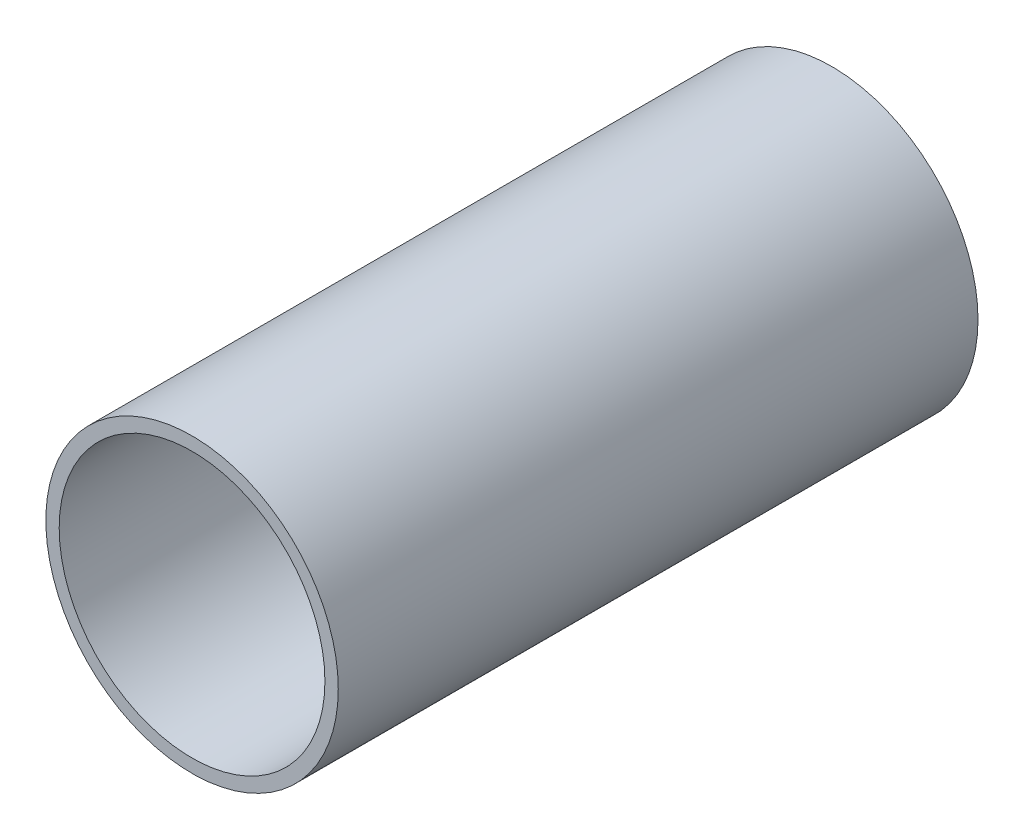
SolidWorks part; units mm, degrees
material "SPHC"
ref_plane "Front Plane" through (0, 0, 0) normal (0, 0, 1) x (1, 0, 0)
ref_plane "Top Plane" through (0, 0, 0) normal (0, 1, 0) x (1, 0, 0)
ref_plane "Right Plane" through (0, 0, 0) normal (1, 0, 0) x (0, 0, -1)
sketch "Sketch1" plane through (0, 0, 0) normal (0, 0, 1) x (1, 0, 0)
  circle A0 centre (0, 0) radius 28.5
  dimension "D1" = 57
extrude "Extrude-Thin1" add sketch "Sketch1" along normal blind 124.7 thin thin type one direction reverse wall 2.6
